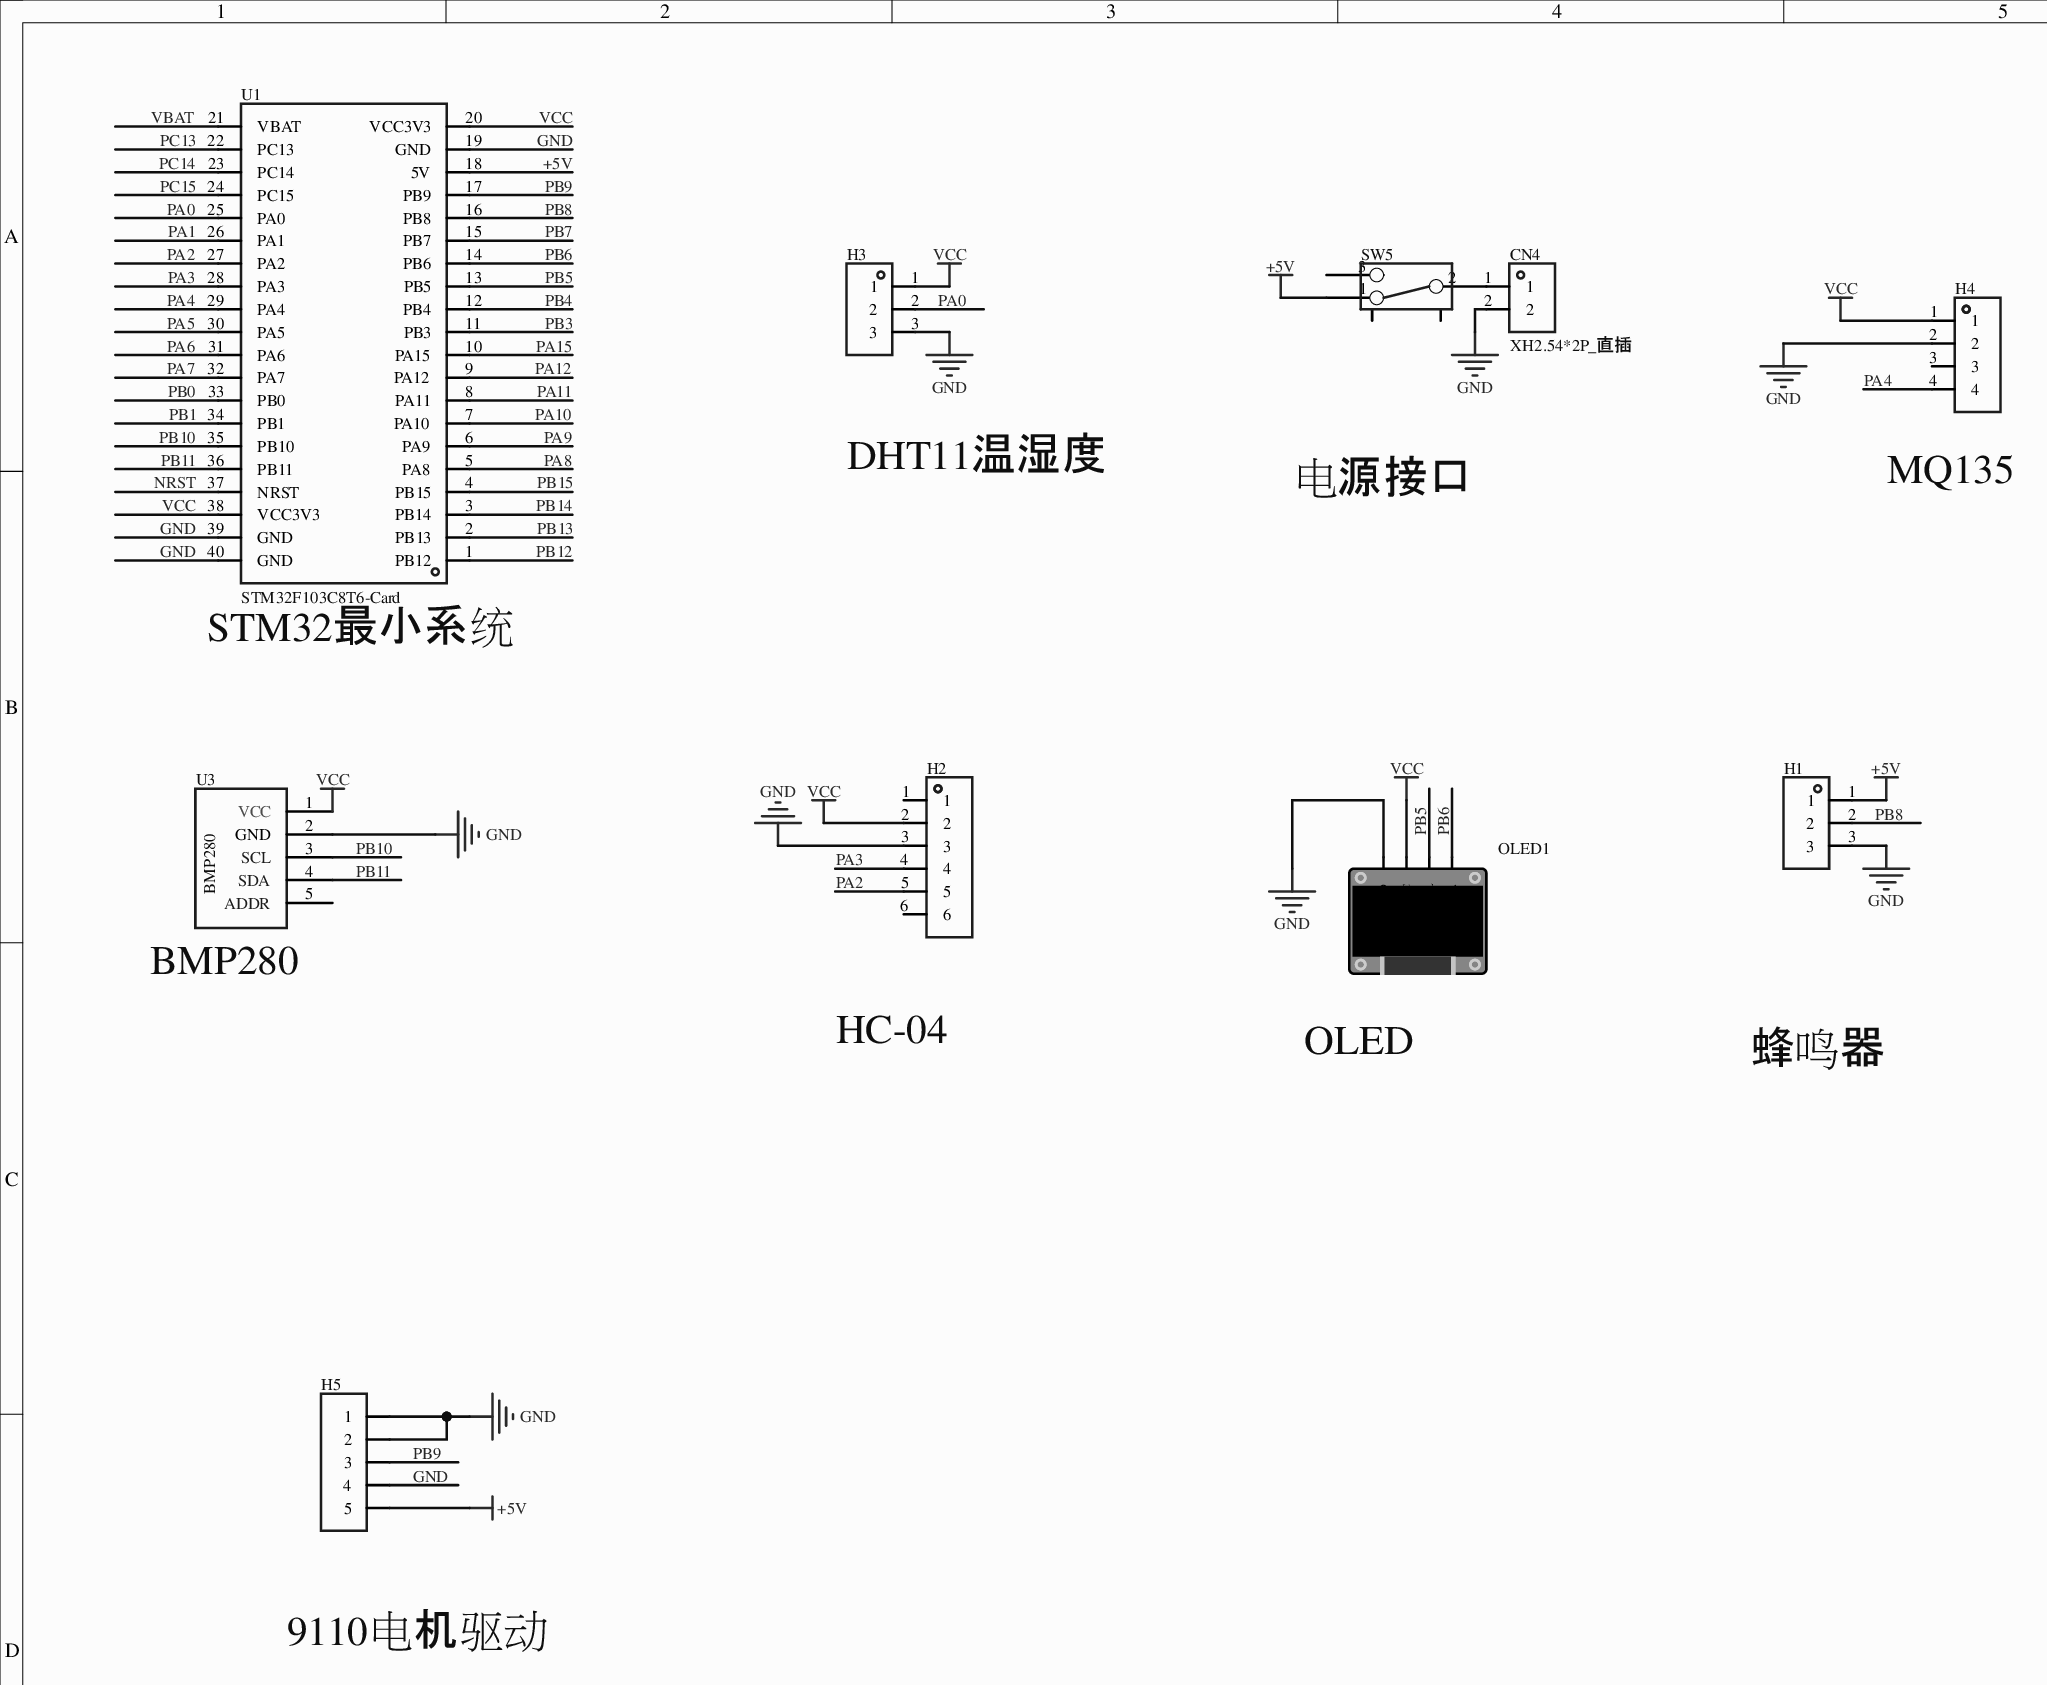
[diagram p0: MISC51936-3.schdoc]
# Altium project MISC51936-2.PrjPcb
1 sheet, 10 parts. Net scope: global (net labels, ports and power ports of the same name join across sheets).
Board file: MISC51936.pcbdoc

## Sheet MISC51936-3.schdoc
size 297 x 209 mm; Version: V1.0; @Project Name: MISC51936; @Page Count: 1; @Update Date: 2026-04-16; @Create Date: 2026-04-16; @Schematic Name: MISC51936; @Page No: 1; @Create Time: 23:22:16; @Update Time: 17:32:40; @Board Name: MISC51936

### Parts
CN4  XH2.54*2P_直插  [CONN-TH_2P-P2.50-XH2.54-2P]
H1  (no value)  [HDR-TH_3P-P2.54-V-F]
H2  (no value)  [HDR-TH_6P-P2.54-V-F]
H3  (no value)  [HDR-TH_3P-P2.54-V-F]
H4  (no value)  [HDR-TH_4P-P2.54-V-F]
H5  (no value)  [HDR-TH_5P-P2.54-V-F]
OLED1  (no value)  [0.96OLED_4P]
SW5  (no value)  [拨动开关]
U1  STM32F103C8T6-Card  [CONN-TH_L53.3-W22.9_STM32F103C8T6-CARD]
U3  (no value)  [BH1750光照传感器]

### Nets
+5V: H1.1 H5.5 SW5.1 U1.18(5V)
GND: CN4.2 H1.3 H2.3 H3.3 H4.2 H5.1 H5.2 H5.4 OLED1.1(GND) U1.19(GND) U1.39(GND) U1.40(GND) U3.2(GND)
VCC: H2.2 H3.1 H4.1 OLED1.2(VCC) U1.20(VCC3V3) U1.38(VCC3V3) U3.1(VCC)
NRST: U1.37(NRST)
PA0: H3.2 U1.25(PA0)
PA1: U1.26(PA1)
PA2: H2.5 U1.27(PA2)
PA3: H2.4 U1.28(PA3)
PA4: H4.4 U1.29(PA4)
PA5: U1.30(PA5)
PA6: U1.31(PA6)
PA7: U1.32(PA7)
PA8: U1.5(PA8)
PA9: U1.6(PA9)
PA10: U1.7(PA10)
PA11: U1.8(PA11)
PA12: U1.9(PA12)
PA15: U1.10(PA15)
PB0: U1.33(PB0)
PB1: U1.34(PB1)
PB3: U1.11(PB3)
PB4: U1.12(PB4)
PB5: OLED1.3(SCL) U1.13(PB5)
PB6: OLED1.4(SDA) U1.14(PB6)
PB7: U1.15(PB7)
PB8: H1.2 U1.16(PB8)
PB9: H5.3 U1.17(PB9)
PB10: U1.35(PB10) U3.3(SCL)
PB11: U1.36(PB11) U3.4(SDA)
PB12: U1.1(PB12)
PB13: U1.2(PB13)
PB14: U1.3(PB14)
PB15: U1.4(PB15)
PC13: U1.22(PC13)
PC14: U1.23(PC14)
PC15: U1.24(PC15)
VBAT: U1.21(VBAT)
NetCN4_1: CN4.1 SW5.2

Not connected (* = marked no-connect by the designer): H2 1 6; H4 3; SW5 3 4 5; U3 5(ADDR)

### Notes on the sheet
- DHT11温湿度
- 电源接口
- (near H4) MQ135
- (near U1) STM32最小系统
- (near U3) BMP280
- HC-04
- OLED
- 蜂鸣器
- 9110电机驱动

### Library data of the parts
CN4 = XH2.54*2P_直插: 3D Model: 325c595e30db4df8abe76612dd40b0fa0819f05c4eef4c71ace90d822a990e87; 3D Model Transform: 295.275,228.346,0,180,0,0,-0.002,-20.079,-137.795; AddInBom: yes; Device: XH2.54*2P_直插; Symbol: XH2.54*2P_直插; LCSC Part Name: XH2.54*2P_直插; Supplier Part: C9900008615; Manufacturer Part: XH2.54*2P_直插; Supplier Footprint: XH2.54_2P; JLCPCB Part Class: Extended Part; Supplier: LCSC; FootprintName: CONN-TH_2P-P2.50-XH2.54-2P; ConvertToPcb: yes; ModelName: CONN-TH_2P-P2.50-XH2.54-2P
H1 H3 = HDR-F_2.54_1x3P: Symbol: PM254V-11-03-H85; 3D Model: f3b3cc5aae9641bf9e56fc160cef875b; 3D Model Transform: 299.9994,100,0,0,0,0,0,0,-118.11; ConvertToPcb: yes; ModelName: HDR2.54-F-LI-1X3P; Device: HDR-F_2.54_1x3P; Supplier Part: C541850; Supplier Footprint: 插件; FootprintName: HDR-TH_3P-P2.54-V-F; AddInBom: yes
H2 = HDR-F_2.54_1x6P: Symbol: Header-Female-2.54_1x6; ConvertToPcb: yes; ModelId: 0f5bcf94dcda47d085f24cdca1696fe9; ModelTransform: 619.684,94.488,0,0,0,0,0,0,-125.984; Device: HDR-F_2.54_1x6P; AddInBom: yes; SupplierPart: C40877; Supplier Footprint: 插件; FootprintName: HDR-TH_6P-P2.54-V-F; ModelName: HDR-TH_6P-P2.54-V-F
H4 = HDR-F_2.54_1x4P: Symbol: 2.54-1*4P母; ConvertToPcb: yes; ModelId: d187812051054f85879fcaa51a310d8e0819f05c4eef4c71ace90d822a990e87; ModelTransform: 419.6842,98.464,0,0,0,0,0,0,-118.11; Device: HDR-F_2.54_1x4P; FootprintName: HDR-TH_4P-P2.54-V-F; AddInBom: yes; SupplierPart: C2718488; Supplier Footprint: 插件; ModelName: HDR-TH_4P-P2.54-V-F
H5 = HDR-F_2.54_1x5P: Symbol: Header-Female-2.54_1x5; ConvertToPcb: yes; ModelId: f49cb6116a3d45e5a64915bf3e00773f; ModelTransform: 519.684,98.464,0,0,0,0,0,0,-124.016; Device: HDR-F_2.54_1x5P; AddInBom: yes; SupplierPart: C50950; Supplier Footprint: 插件; FootprintName: HDR-TH_5P-P2.54-V-F; ModelName: HDR-TH_5P-P2.54-V-F
OLED1 = 0.96OLED模块_4P: ConvertToPcb: yes; ModelId: 79c000fdb68d45a296c2e9bedf4f9055; ModelTransform: 1393.69792,1318.895,0,0,0,0,0,-560.079,-137.795; Symbol: 0.96OLED模块_4P; Device: 0.96OLED模块_4P; AddInBom: yes; FootprintName: 0.96OLED_4P; Supplier Footprint: 插件; ModelName: 0.96OLED_4P
SW5 = 拨动开关_正: ConvertToPcb: yes; ModelId: 4321fe59a4074cbfb4989553f297c68f0819f05c4eef4c71ace90d822a990e87; ModelName: SW-TH_SS-12D02-VG4; ModelTransform: 370.09,208.7,472.35,0,0,0,0,0,-110; Device: 拨动开关_正; Symbol: 拨动开关; FootprintName: 拨动开关; AddInBom: yes; Supplier Footprint: 插件
U1 = STM32F103C8T6-Card: AddInBom: yes; Device: STM32F103C8T6-Card; Symbol: STM32F103C8T6-CARD; FootprintName: CONN-TH_L53.3-W22.9_STM32F103C8T6-CARD; LCSC Part Name: STM32F103C8T6-Card; SupplierPart: C9900077949; ManufacturerPart: STM32F103C8T6-Card; Supplier Footprint: 插件; Supplier: LCSC; ConvertToPcb: yes
U3 = BH1750光照传感器: Symbol: BH1750光照传感器_1; AddInBom: yes; Device: BH1750光照传感器; ConvertToPcb: yes; FootprintName: BH1750光照传感器